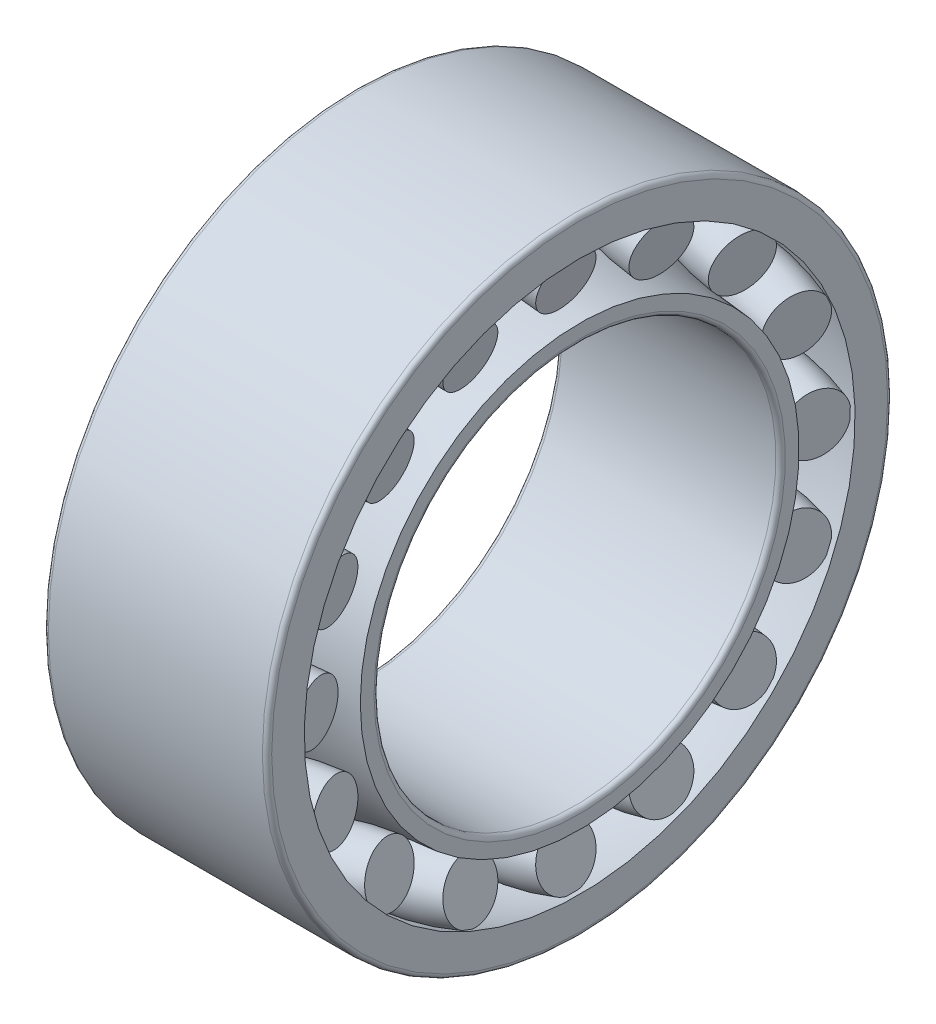
SolidWorks part; units mm, degrees
ref_plane "Front" through (0, 0, 0) normal (0, 0, 1) x (1, 0, 0)
ref_plane "Top" through (0, 0, 0) normal (0, 1, 0) x (1, 0, 0)
ref_plane "Right" through (0, 0, 0) normal (1, 0, 0) x (0, 0, -1)
other "Configuration Table"
sketch "Sketch1" plane through (0, 0, 0) normal (0, 0, 1) x (1, 0, 0)
  line L0 (-50, 0) -> (50, 0) construction
  line L1 (50, 123.3333) -> (50, 140)
  line L2 (-8.3333, 106.6667) -> (8.3333, 106.6667)
  line L3 (-50, 90) -> (50, 90)
  line L4 (-50, 90) -> (-50, 98.2402)
  line L5 (-50, 140) -> (50, 140)
  line L6 (50, 90) -> (50, 98.2402)
  line L7 (0, 0) -> (0, 140) construction
  line L8 (-50, 123.3333) -> (-50, 140)
  line L9 (-8.3333, 106.6667) -> (-14.4528, 132.296)
  line L10 (-46.8747, 124.5547) -> (-40.7553, 98.9254)
  line L11 (8.3333, 106.6667) -> (14.4528, 132.296)
  line L12 (46.8747, 124.5547) -> (40.7553, 98.9254)
  line L13 (14.4528, 115) -> (50, 115)
  line L14 (-42.6037, 106.6667) -> (-50, 106.6667)
  line L15 (-43.815, 111.74) -> (-11.3931, 119.4813)
  line L16 (-49.98, 123.363) -> (-49.98, 139.98)
  line L17 (-49.98, 139.98) -> (49.98, 139.98)
  line L18 (49.98, 123.363) -> (49.98, 139.98)
  line L19 (-49.98, 90.02) -> (-49.98, 98.221)
  line L20 (-49.98, 90.02) -> (49.98, 90.02)
  line L21 (49.98, 90.02) -> (49.98, 98.221)
  arc A0 (50, 123.3333) -> (-50, 123.3333) centre (0, 0) ccw
  arc A1 (-8.3333, 106.6667) -> (-50, 98.2402) centre (-55.2081, 231.2214) cw
  arc A2 (8.3333, 106.6667) -> (50, 98.2402) centre (55.2081, 231.2214) ccw
  arc A3 (49.98, 123.363) -> (-49.98, 123.363) centre (0, 0) ccw
  arc A4 (-19.8326, 102.9053) -> (-49.98, 98.221) centre (-55.2081, 231.2214) cw
  arc A5 (19.8326, 102.9053) -> (49.98, 98.221) centre (55.2081, 231.2214) ccw
  point P16 (0, 140)
revolve "Revolve1" add sketch "Sketch1" angle 360 about L0
sketch "Sketch2" plane through (0, 0, 0) normal (0, 0, 1) x (1, 0, 0)
  line L0 (-8.3333, 106.6667) -> (-14.4528, 132.296) construction
  line L1 (-43.815, 111.74) -> (-11.3931, 119.4813) construction
  line L2 (-46.8747, 124.5547) -> (-40.7553, 98.9254) construction
  line L3 (-11.3931, 119.4813) -> (-14.4528, 132.296)
  line L4 (-43.815, 111.74) -> (-11.3931, 119.4813)
  line L5 (-46.8747, 124.5547) -> (-43.815, 111.74)
  line L6 (-43.815, 111.74) -> (-12.9279, 119.1149) construction
  arc A0 (50, 123.3333) -> (-50, 123.3333) centre (0, 0) ccw construction
  arc A1 (-14.4528, 132.296) -> (-46.8747, 124.5547) centre (0, 0) ccw
revolve "Revolve2" add sketch "Sketch2" angle 360 about L6
sketch "Sketch3" plane through (0, 0, 0) normal (0, 0, 1) x (1, 0, 0)
  line L0 (-50, 123.3333) -> (-50, 140) construction
  line L1 (50, 123.3333) -> (50, 140) construction
  line L2 (-50, 140) -> (50, 140) construction
  line L3 (-50, 123.3333) -> (-50, 140)
  line L4 (50, 123.3333) -> (50, 140)
  line L5 (-50, 140) -> (50, 140)
  arc A0 (50, 123.3333) -> (-50, 123.3333) centre (0, 0) ccw construction
  arc A1 (50, 123.3333) -> (-50, 123.3333) centre (0, 0) ccw
revolve "Revolve3" add sketch "Sketch3" angle 360 about axis through (-50, 0, 0) along (1, 0, 0)
mirror "Mirror1" about plane through (0, 0, 0) normal (1, 0, 0) of bodies 102
pattern_circular "Circular-Pattern1" count 16 over 360 about axis through (0, 0, 0) along (1, 0, 0) of bodies 105 102
fillet "Fillet1" radius 2.1 2 edges at (-50, 0, 140) (50, 0, 140)
fillet "Fillet2" radius 2.1 2 edges at (50, 0, 90) (-50, 0, 90)
sketch "Sketch4" plane through (0, 0, 0) normal (0, 0, 1) x (1, 0, 0)
  line L0 (-46.8747, 124.5547) -> (-40.7553, 98.9254) construction
  line L1 (-42.6037, 106.6667) -> (-50, 106.6667) construction
  line L2 (-42.6037, 106.6667) -> (-40.7553, 98.9254)
  line L3 (-42.6037, 106.6667) -> (-50, 106.6667)
  line L4 (-50, 106.6667) -> (-50, 98.2402)
  arc A0 (-50, 98.2402) -> (-8.3333, 106.6667) centre (-55.2081, 231.2214) ccw construction
  arc A1 (-50, 98.2402) -> (-40.7553, 98.9254) centre (-55.2081, 231.2214) ccw
revolve "Revolve4" [suppressed] add sketch "Sketch4" angle 360 about axis through (-50, 0, 0) along (1, 0, 0)
mirror "Mirror2" [suppressed] about plane through (0, 0, 0) normal (1, 0, 0)
equation "\"D1@Fillet2\"=\"D1@Fillet1\""
equation "\"XD1@Sketch1\" =  ( 2 * \"XD@Sketch1\" + \"DD@Sketch1\" )  /3"
equation "\"DD1@Sketch1\" =  ( 2 * \"DD@Sketch1\" + \"XD@Sketch1\" )  / 3"
equation "\"GZJJ@Sketch1\" = \"DB@Sketch1\" / 6"
equation "\"GZK@Sketch1\" = \"DB@Sketch1\" / 3"
equation "\"zj@Sketch1\" = (  \"DD@Sketch1\" + \"XD@Sketch1\" )  / 2"
equation "\"D1@Circular-Pattern1\" = int( 3.14159265 / atn(( \"GZK@Sketch1\" / 2) / sqr( \"XD@Sketch1\" * \"XD@Sketch1\"/4 - ( \"GZK@Sketch1\" / 2) *  ( \"GZK@Sketch1\" / 2))))"
equation "\"D1@Sketch1\" = \"XD1@Sketch1\" + 0.002"
